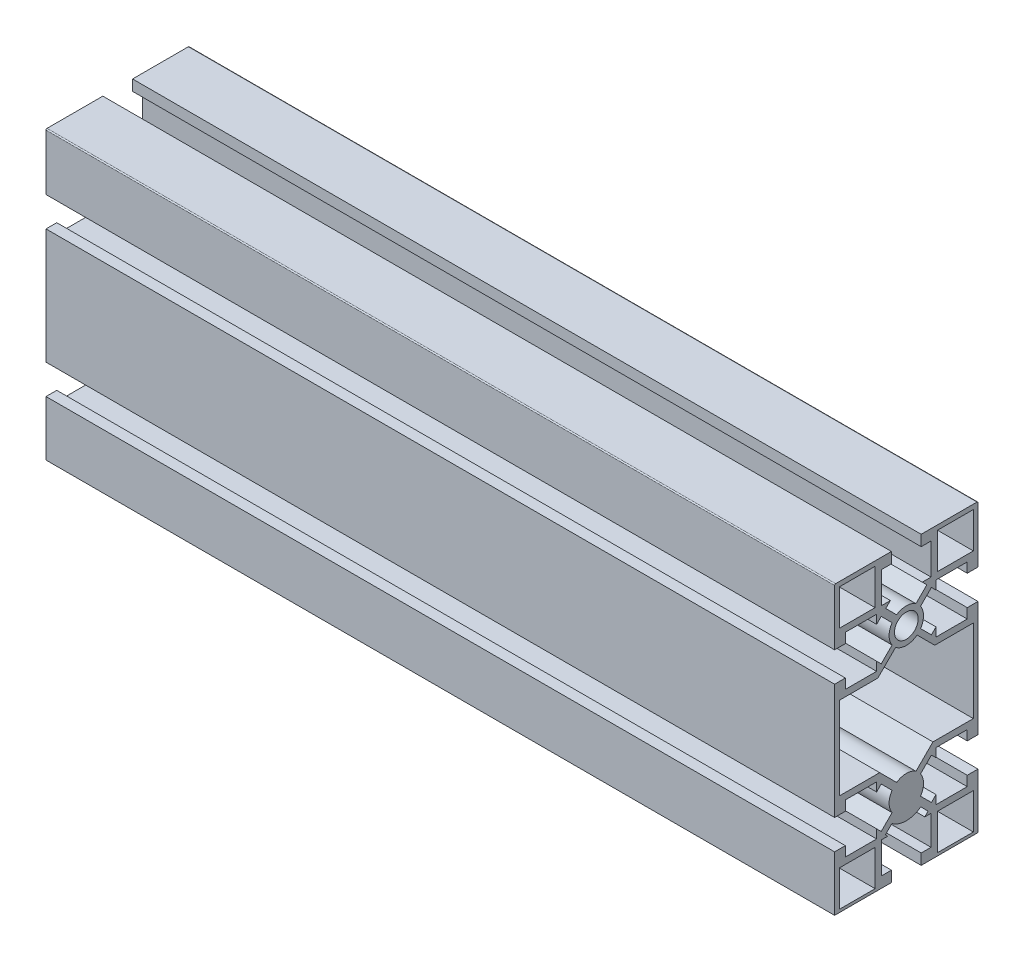
from build123d import *

# Parameters (mm, degrees)
SKETCH13_R                               = 3.3
SKETCH13_W                               = 10
SKETCH13_H                               = 10
ALUMINUM_PROFILE_40_X_80L_X_R0_3_1_DEPTH = 220


with BuildPart() as part:
    # Sketch13 → Aluminum profile 40 X 80L X R0.3(1) (new body)
    with BuildSketch(Plane(origin=(-251.127596439, 0, 4.629080119), x_dir=(0, 0, -1), z_dir=(1, 0, 0))):
        with BuildLine():
            Line((-19.7, 20), (-4.15, 20))
            Line((-4.15, 20), (-4.15, 17))
            Line((-4.15, 17), (-6.9, 17))
            Line((-6.9, 17), (-6.9, 8.28356292))
            Line((-6.9, 8.28356292), (-4.444359142, 8.28356292))
            Line((-4.444359142, 8.28356292), (-5.727564928, 7.000357134))
            Line((-5.727564928, 7.000357134), (-2.697520513, 3.970312719))
            ThreePointArc((-2.697520513, 3.970312719), (0, 4.8), (2.697520513, 3.970312719))
            Line((2.697520513, 3.970312719), (5.727564928, 7.000357134))
            Line((5.727564928, 7.000357134), (4.444359142, 8.28356292))
            Line((4.444359142, 8.28356292), (6.9, 8.28356292))
            Line((6.9, 8.28356292), (6.9, 17))
            Line((6.9, 17), (4.15, 17))
            Line((4.15, 17), (4.15, 20))
            Line((4.15, 20), (19.7, 20))
            ThreePointArc((19.7, 20), (19.912132034, 19.912132034), (20, 19.7))
            Line((20, 19.7), (20, 4.15))
            Line((20, 4.15), (17, 4.15))
            Line((17, 4.15), (17, 6.9))
            Line((17, 6.9), (8.28356292, 6.9))
            Line((8.28356292, 6.9), (8.28356292, 4.444359142))
            Line((8.28356292, 4.444359142), (7.000357134, 5.727564928))
            Line((7.000357134, 5.727564928), (3.970312719, 2.697520513))
            ThreePointArc((3.970312719, 2.697520513), (4.8, 0), (3.970312719, -2.697520513))
            Line((3.970312719, -2.697520513), (7.000357134, -5.727564928))
            Line((7.000357134, -5.727564928), (8.28356292, -4.444359142))
            Line((8.28356292, -4.444359142), (8.28356292, -6.9))
            Line((8.28356292, -6.9), (17, -6.9))
            Line((17, -6.9), (17, -4.15))
            Line((17, -4.15), (20, -4.15))
            Line((20, -4.15), (20, -36.35))
            Line((20, -36.35), (17, -36.35))
            Line((17, -36.35), (17, -33.6))
            Line((17, -33.6), (8.28356292, -33.6))
            Line((8.28356292, -33.6), (8.28356292, -36.055640858))
            Line((8.28356292, -36.055640858), (7.000357134, -34.772435072))
            Line((7.000357134, -34.772435072), (3.970312719, -37.802479487))
            ThreePointArc((3.970312719, -37.802479487), (4.8, -40.5), (3.970312719, -43.197520513))
            Line((3.970312719, -43.197520513), (7.000357134, -46.227564928))
            Line((7.000357134, -46.227564928), (8.28356292, -44.944359142))
            Line((8.28356292, -44.944359142), (8.28356292, -47.4))
            Line((8.28356292, -47.4), (17, -47.4))
            Line((17, -47.4), (17, -44.65))
            Line((17, -44.65), (20, -44.65))
            Line((20, -44.65), (20, -60))
            Line((20, -60), (4.15, -60))
            Line((4.15, -60), (4.15, -57))
            Line((4.15, -57), (6.9, -57))
            Line((6.9, -57), (6.9, -48.78356292))
            Line((6.9, -48.78356292), (5.151465923, -48.78356292))
            Line((5.151465923, -48.78356292), (6.081118318, -47.853910524))
            Line((6.081118318, -47.853910524), (4.02260057, -45.795392776))
            ThreePointArc((4.02260057, -45.795392776), (0, -47.15), (-4.02260057, -45.795392776))
            Line((-4.02260057, -45.795392776), (-5.831118318, -47.603910524))
            Line((-5.831118318, -47.603910524), (-5.151465923, -48.28356292))
            Line((-5.151465923, -48.28356292), (-6.9, -48.28356292))
            Line((-6.9, -48.28356292), (-6.9, -57))
            Line((-6.9, -57), (-4.15, -57))
            Line((-4.15, -57), (-4.15, -60))
            Line((-4.15, -60), (-20, -60))
            Line((-20, -60), (-20, -44.65))
            Line((-20, -44.65), (-17, -44.65))
            Line((-17, -44.65), (-17, -47.4))
            Line((-17, -47.4), (-8.28356292, -47.4))
            Line((-8.28356292, -47.4), (-8.28356292, -44.944359142))
            Line((-8.28356292, -44.944359142), (-7.000357134, -46.227564928))
            Line((-7.000357134, -46.227564928), (-3.970312719, -43.197520513))
            ThreePointArc((-3.970312719, -43.197520513), (-4.8, -40.5), (-3.970312719, -37.802479487))
            Line((-3.970312719, -37.802479487), (-7.000357134, -34.772435072))
            Line((-7.000357134, -34.772435072), (-8.28356292, -36.055640858))
            Line((-8.28356292, -36.055640858), (-8.28356292, -33.6))
            Line((-8.28356292, -33.6), (-17, -33.6))
            Line((-17, -33.6), (-17, -36.35))
            Line((-17, -36.35), (-20, -36.35))
            Line((-20, -36.35), (-20, -4.15))
            Line((-20, -4.15), (-17, -4.15))
            Line((-17, -4.15), (-17, -6.9))
            Line((-17, -6.9), (-8.28356292, -6.9))
            Line((-8.28356292, -6.9), (-8.28356292, -4.444359142))
            Line((-8.28356292, -4.444359142), (-7.000357134, -5.727564928))
            Line((-7.000357134, -5.727564928), (-3.970312719, -2.697520513))
            ThreePointArc((-3.970312719, -2.697520513), (-4.8, 0), (-3.970312719, 2.697520513))
            Line((-3.970312719, 2.697520513), (-7.000357134, 5.727564928))
            Line((-7.000357134, 5.727564928), (-8.28356292, 4.444359142))
            Line((-8.28356292, 4.444359142), (-8.28356292, 6.9))
            Line((-8.28356292, 6.9), (-17, 6.9))
            Line((-17, 6.9), (-17, 4.15))
            Line((-17, 4.15), (-20, 4.15))
            Line((-20, 4.15), (-20, 19.7))
            ThreePointArc((-20, 19.7), (-19.912132034, 19.912132034), (-19.7, 20))
        make_face()
        Circle(SKETCH13_R, mode=Mode.SUBTRACT)
        with BuildLine():
            Line((-18.7, -8.7), (-18.7, -31.8))
            Line((-18.7, -31.8), (-7.427207794, -31.8))
            Line((-7.427207794, -31.8), (-2.697520513, -36.529687281))
            ThreePointArc((-2.697520513, -36.529687281), (0, -35.7), (2.697520513, -36.529687281))
            Line((2.697520513, -36.529687281), (7.427207794, -31.8))
            Line((7.427207794, -31.8), (18.7, -31.8))
            Line((18.7, -31.8), (18.7, -8.7))
            Line((18.7, -8.7), (7.927207794, -8.7))
            Line((7.927207794, -8.7), (2.985650464, -3.75844267))
            ThreePointArc((2.985650464, -3.75844267), (0, -4.8), (-2.985650464, -3.75844267))
            Line((-2.985650464, -3.75844267), (-7.927207794, -8.7))
            Line((-7.927207794, -8.7), (-18.7, -8.7))
        make_face(mode=Mode.SUBTRACT)
        with Locations((-13.7, 13.7)):
            Rectangle(SKETCH13_W, SKETCH13_H, mode=Mode.SUBTRACT)
        with Locations((13.7, 13.7)):
            Rectangle(SKETCH13_W, SKETCH13_H, mode=Mode.SUBTRACT)
        with Locations((-13.7, -54.2)):
            Rectangle(SKETCH13_W, SKETCH13_H, mode=Mode.SUBTRACT)
        with Locations((13.7, -54.2)):
            Rectangle(SKETCH13_W, SKETCH13_H, mode=Mode.SUBTRACT)
    extrude(amount=ALUMINUM_PROFILE_40_X_80L_X_R0_3_1_DEPTH)


solid = part.part
